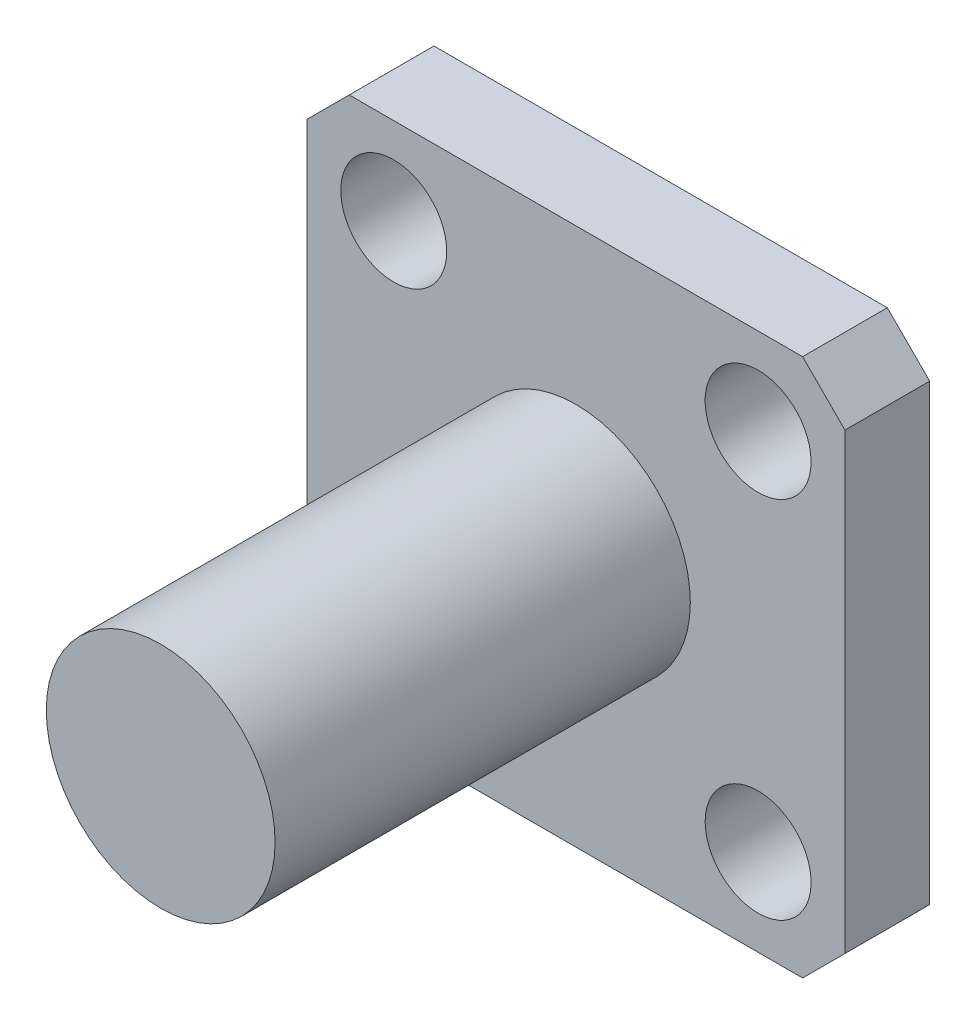
from build123d import *

# Parameters (mm, degrees)
SKETCH1_W           = 12.7
SKETCH1_H           = 12.7
SKETCH1_R           = 1.25
BOSS_EXTRUDE1_DEPTH = 2
CHAMFER1_SIZE       = 1
SKETCH2_R           = 2.7
BOSS_EXTRUDE2_DEPTH = 4.6
SKETCH3_R           = 2.7
BOSS_EXTRUDE3_DEPTH = 5.2


with BuildPart() as part:
    # Sketch1 → Boss-Extrude1 (new body)
    with BuildSketch(Plane.XY):
        with Locations((-6.35, -6.35)):
            Rectangle(SKETCH1_W, SKETCH1_H)
        with Locations((-10.65, -2.05)):
            Circle(SKETCH1_R, mode=Mode.SUBTRACT)
        with Locations((-2.05, -2.05)):
            Circle(SKETCH1_R, mode=Mode.SUBTRACT)
        with Locations(Location((-2.05, -10.65, 0), (0, 0, 180))):
            Circle(SKETCH1_R, mode=Mode.SUBTRACT)
        with Locations(Location((-10.65, -10.65, 0), (0, 0, 180))):
            Circle(SKETCH1_R, mode=Mode.SUBTRACT)
    extrude(amount=BOSS_EXTRUDE1_DEPTH)

    # Chamfer1
    chamfer1_edges = [part.edges().sort_by_distance(p)[0] for p in [
        (0, -12.7, 1),
        (-12.7, -12.7, 1),
        (-12.7, 0, 1),
        (0, 0, 1),
    ]]
    chamfer(chamfer1_edges, length=CHAMFER1_SIZE)

    # Sketch2 → Boss-Extrude2 (add)
    with BuildSketch(Plane.XY.offset(2)):
        with Locations((-6.35, -6.35)):
            Circle(SKETCH2_R)
    extrude(amount=BOSS_EXTRUDE2_DEPTH)

    # Sketch3 → Boss-Extrude3 (add)
    with BuildSketch(Plane.XY.offset(6.6)):
        with Locations((-6.35, -6.35)):
            Circle(SKETCH3_R)
    extrude(amount=BOSS_EXTRUDE3_DEPTH)


solid = part.part
